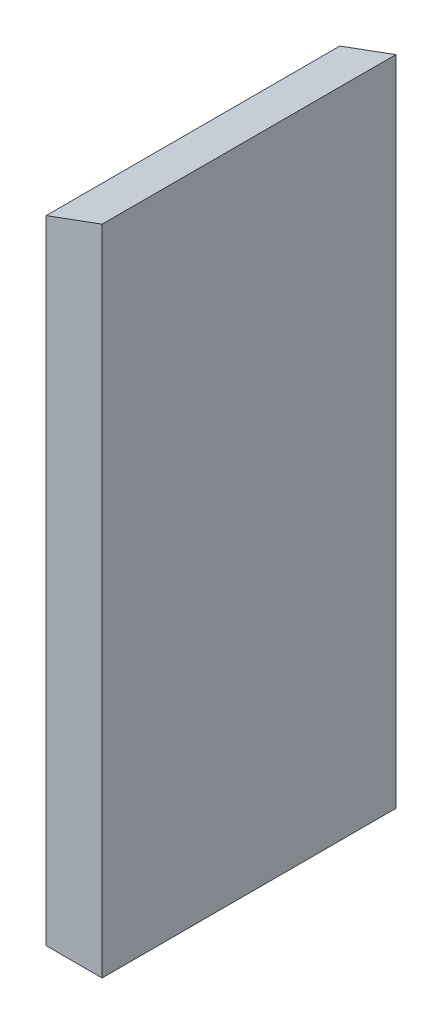
from build123d import *

# Parameters (mm, degrees)
EXTRUDE_1_DEPTH = 25
EXTRUDE_2_DEPTH = 17


with BuildPart() as part:
    # 草图1 → 凸台-拉伸1 (new body)
    with BuildSketch(Plane.XY):
        Polygon((176.477803528, 193), (184.477803528, 193), (184.477803528, 286.35815759), (176.477803528, 283.424824257), align=None)
    extrude(amount=EXTRUDE_1_DEPTH)

    # 草图2 → 凸台-拉伸2 (add)
    with BuildSketch(Plane.XY.offset(25)):
        Polygon((176.477803528, 283.424824257), (176.477803528, 193), (184.477803528, 193), (184.477803528, 286.35815759), align=None)
    extrude(amount=EXTRUDE_2_DEPTH)


solid = part.part
